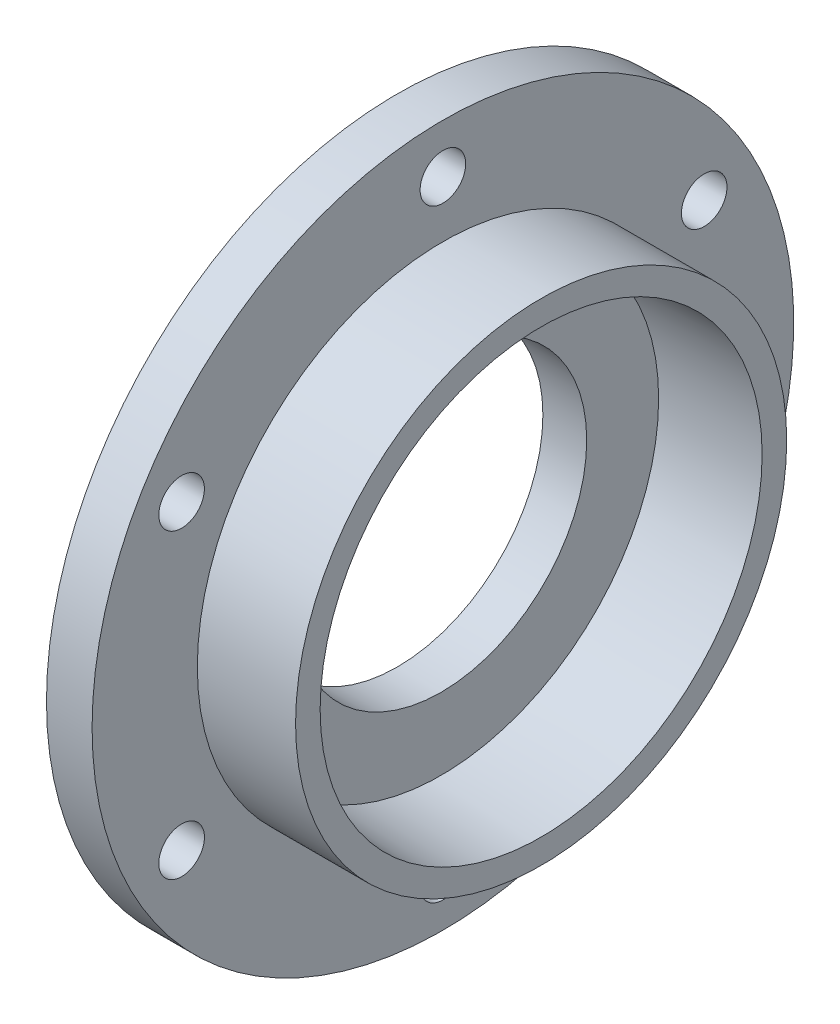
from build123d import *

# Parameters (mm, degrees)
SKETCH2_R          = 6.5
CUT_EXTRUDE1_DEPTH = 145.166570328
CIRPATTERN1_COUNT  = 6
SKETCH3_R          = 41.5
CUT_EXTRUDE2_DEPTH = 148.244694302
DRAFT1_ANGLE       = 2


with BuildPart() as part:
    # Sketch1 → Revolve1 (revolve)
    with BuildSketch(Plane.XY, mode=Mode.PRIVATE) as revolve1_sk:
        Polygon((0, 0), (0, 100), (13, 100), (13, 70), (41, 70), (41, 62), (12.495221111, 62), (12.495221111, 0), align=None)
    revolve(revolve1_sk.sketch.rotate(Axis((0, 0, 0), (1, 0, 0)), 90), axis=Axis((0, 0, 0), (1, 0, 0)))

    # Sketch2 → Cut-Extrude1 (cut, through all)
    with BuildSketch(Plane(origin=(13, 0, 0), x_dir=(0, 0, -1), z_dir=(1, 0, 0))):
        with Locations((0, 86)):
            Circle(SKETCH2_R)
    cut_extrude1 = extrude(amount=-CUT_EXTRUDE1_DEPTH, mode=Mode.SUBTRACT)

    # CirPattern1: Cut-Extrude1 ×6 about axis
    cirpattern1_axis = Axis((0, 0, 0), (1, 0, 0))
    for i in range(1, CIRPATTERN1_COUNT):
        add(cut_extrude1.rotate(cirpattern1_axis, i * 360 / CIRPATTERN1_COUNT), mode=Mode.SUBTRACT)

    # Sketch3 → Cut-Extrude2 (cut, through all)
    with BuildSketch(Plane.ZY):
        Circle(SKETCH3_R)
    extrude(amount=-CUT_EXTRUDE2_DEPTH, mode=Mode.SUBTRACT)

    # Draft1
    draft1_faces = [part.faces().sort_by_distance(p)[0] for p in [
        (26.747610556, 0, -62),
    ]]
    draft(draft1_faces, Plane(origin=(12.495221111, 62, 0), x_dir=(0, 0, 1), z_dir=(1, 0, 0)), DRAFT1_ANGLE)


solid = part.part
